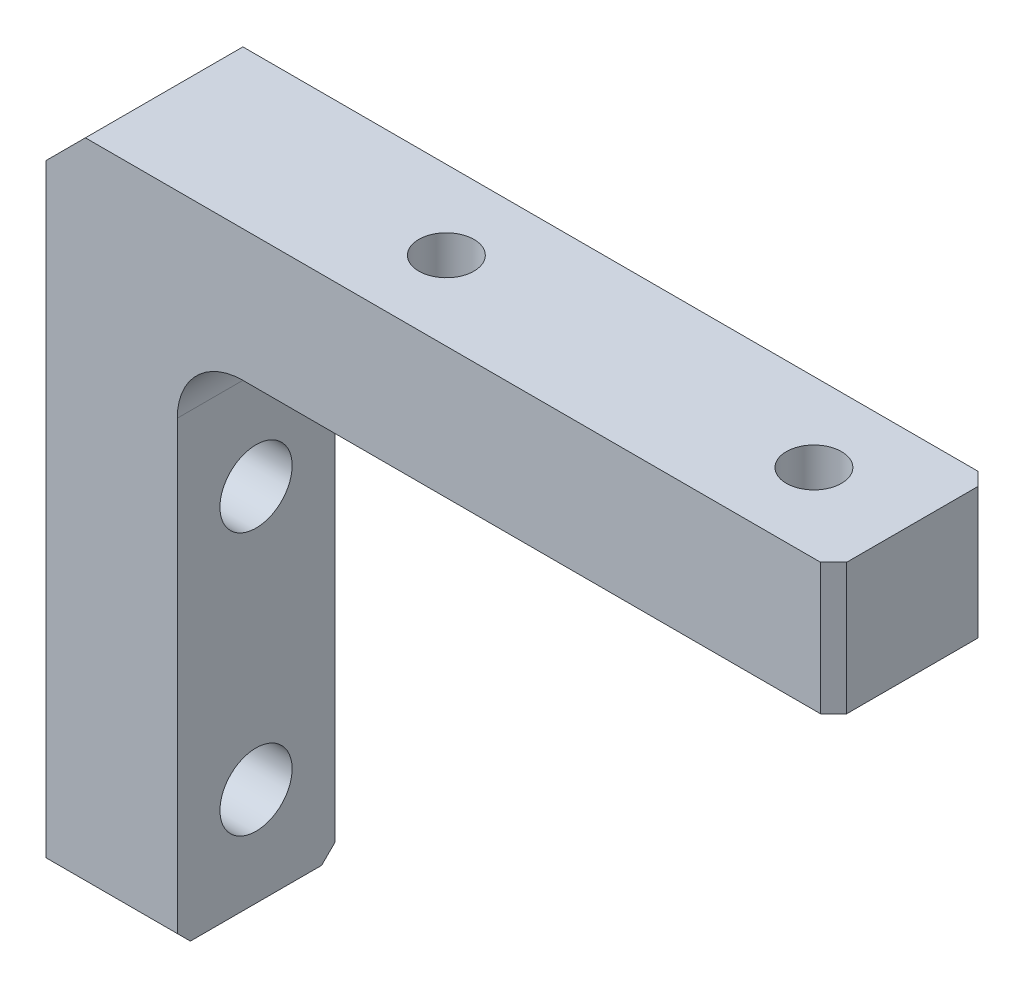
SolidWorks part; units mm, degrees
material "AL6061"
ref_plane "Front Plane" through (0, 0, 0) normal (0, 0, 1) x (1, 0, 0)
ref_plane "Top Plane" through (0, 0, 0) normal (0, 1, 0) x (1, 0, 0)
ref_plane "Right Plane" through (0, 0, 0) normal (1, 0, 0) x (0, 0, -1)
sketch "Sketch1" plane through (0, 0, 0) normal (0, 0, 1) x (1, 0, 0)
  line L0 (3, 0) -> (60, 0)
  line L2 (0, -50) -> (0, -3)
  line L3 (0, -50) -> (10, -50)
  line L5 (60, -10) -> (60, 0)
  line L6 (10, -50) -> (10, -10)
  line L7 (10, -10) -> (60, -10)
  line L8 (3, 0) -> (0, -3)
  dimension "D1" = 3
  dimension "D2" = 3
  dimension "D3" = 10
  dimension "D4" = 10
  dimension "D5" = 60
  dimension "D6" = 50
extrude "Boss-Extrude1" add sketch "Sketch1" along normal blind 12
hole_wizard "M5 Tapped Hole1" positions "Sketch4" profile "Sketch5" tap size "M5" standard "GB"
sketch "Sketch4" plane through (0, 0, 0) normal (0, -1, 0) x (-1, 0, 0)
  line L0 (-60, -6) -> (0, -6) construction
  line L1 (-60, -12) -> (-60, 0) construction
  line L3 (0, -12) -> (0, 0) construction
  point P0 (-52.5, -6)
  point P15 (-24.5, -6)
  dimension "D1" = 7.5
  dimension "D2" = 28
sketch "Sketch5" plane through (52.5, 0, 6) normal (1, 0, 0) x (0, 0, 1)
  line L0 (0, 0) -> (0, 13.6618)
  line L1 (0, 13.6618) -> (2.1, 12.4)
  line L2 (2.1, 12.4) -> (2.1, 0)
  line L5 (2.1, 0) -> (0, 0)
  line L10 (0, 13.6618) -> (-2.1, 12.4) construction
  line L11 (0, -6.35) -> (0, 107.95) construction
  dimension "螺纹孔钻头直径" = 4.2
  dimension "螺纹孔钻头深度" = 12.4
  dimension "导头角度" = 118
hole_wizard "M5 Clearance Hole1" positions "Sketch6" profile "Sketch7" hole size "M5" standard "GB" end condition through all
sketch "Sketch6" plane through (10, 0, 0) normal (1, 0, 0) x (0, 0, -1)
  line L0 (-6, 0) -> (-6, -50) construction
  line L2 (-12, -50) -> (0, -50) construction
  line L3 (-12, 0) -> (0, 0) construction
  point P0 (-6, -42.5)
  point P17 (-6, -22.5)
  dimension "D1" = 7.5
  dimension "D2" = 20
sketch "Sketch7" plane through (10, -42.5, 6) normal (0, 1, 0) x (0, 0, -1)
  line L0 (0, 0) -> (0, 10)
  line L1 (0, 10) -> (2.75, 10)
  line L2 (2.75, 10) -> (2.75, 0)
  line L5 (2.75, 0) -> (0, 0)
  line L11 (0, -6.35) -> (0, 107.95) construction
  dimension "通孔孔直径" = 5.5
  dimension "通孔孔深度" = 10
chamfer "Chamfer2" distance 1 angle 45 4 edges at (60, -5, 12) (60, -5, 0) (5, -50, 12) (5, -50, 0)
fillet "Fillet1" radius 5 1 edges at (10, -10, 6)
